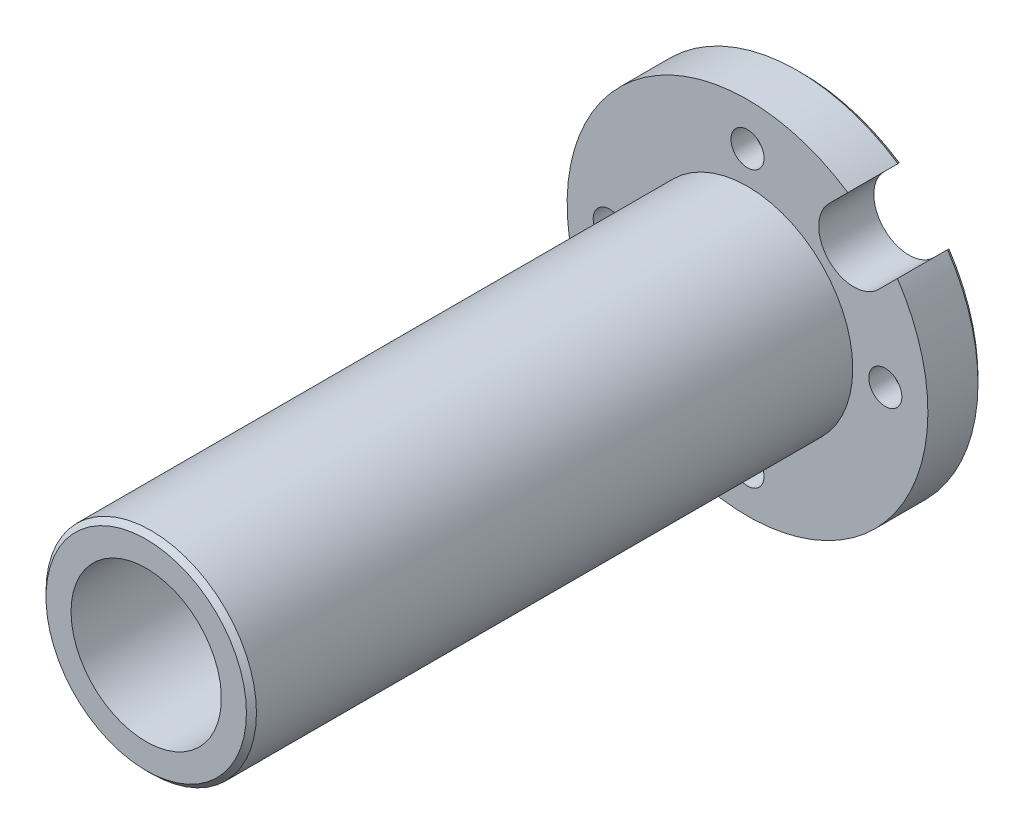
from build123d import *

# Parameters (mm, degrees)
SKETCH_1_W                   = 36
SKETCH_1_H                   = 11
CUT_EXTRUDE_1_DEPTH          = 53.086466572
SKETCH_3_W                   = 21
SKETCH_3_H                   = 120
HOLE_WIZARD_M27_1_D          = 30
HOLE_WIZARD_M6_1_D           = 6.6
HOLE_WIZARD_M6_1_DEPTH       = 131
HOLE_WIZARD_M6_1_CBORE_D     = 11
HOLE_WIZARD_M6_1_CBORE_DEPTH = 6.4
CHAMFER_1_SIZE               = 1


with BuildPart() as part:
    # 草图1 → 旋转1 (revolve)
    with BuildSketch(Plane.XZ, mode=Mode.PRIVATE) as revolve_1_sk:
        with Locations((18, 5.5)):
            Rectangle(SKETCH_1_W, SKETCH_1_H)
    revolve(revolve_1_sk.sketch.rotate(Axis((0, 0, 11), (0, 0, -1)), 180), axis=Axis((0, 0, 11), (0, 0, -1)))

    # 草图2 → 切除-拉伸1 (cut, through all)
    with BuildSketch(Plane.XY.offset(11)):
        with BuildLine():
            Line((20.02023451, 29.919729447), (16.263455967, 26.162950904))
            ThreePointArc((16.263455967, 26.162950904), (16.263455967, 16.263455967), (26.162950904, 16.263455967))
            Line((26.162950904, 16.263455967), (29.919729447, 20.02023451))
            ThreePointArc((29.919729447, 20.02023451), (25.455844123, 25.455844123), (20.02023451, 29.919729447))
        make_face()
    extrude(amount=-CUT_EXTRUDE_1_DEPTH, mode=Mode.SUBTRACT)

    # 草图3 → 旋转2 (revolve)
    with BuildSketch(Plane.XZ, mode=Mode.PRIVATE) as revolve_2_sk:
        with Locations((10.5, 71)):
            Rectangle(SKETCH_3_W, SKETCH_3_H)
    revolve(revolve_2_sk.sketch.rotate(Axis((0, 0, 131), (0, 0, -1)), 180), axis=Axis((0, 0, 131), (0, 0, -1)))

    # M27 间隙孔1 (through all)
    with Locations(Plane(origin=(0, 0, 0), x_dir=(-1, 0, 0), z_dir=(0, 0, -1))):
        with Locations((0, 0)):
            Hole(HOLE_WIZARD_M27_1_D / 2)

    # M6 六角头螺栓的柱形沉头孔1
    with Locations(Plane(origin=(0, 0, 0), x_dir=(-1, 0, 0), z_dir=(0, 0, -1))):
        with Locations((0, 27.5), (27.5, 0), (0, -27.5), (-27.5, 0)):
            CounterBoreHole(HOLE_WIZARD_M6_1_D / 2, HOLE_WIZARD_M6_1_CBORE_D / 2, HOLE_WIZARD_M6_1_CBORE_DEPTH, depth=HOLE_WIZARD_M6_1_DEPTH)

    # 倒角1
    chamfer_1_edges = [part.edges().sort_by_distance(p)[0] for p in [
        (-25.455844123, -25.455844123, 0),
        (21, 0, 131),
        (-15, 0, 0),
    ]]
    chamfer(chamfer_1_edges, length=CHAMFER_1_SIZE)


solid = part.part
